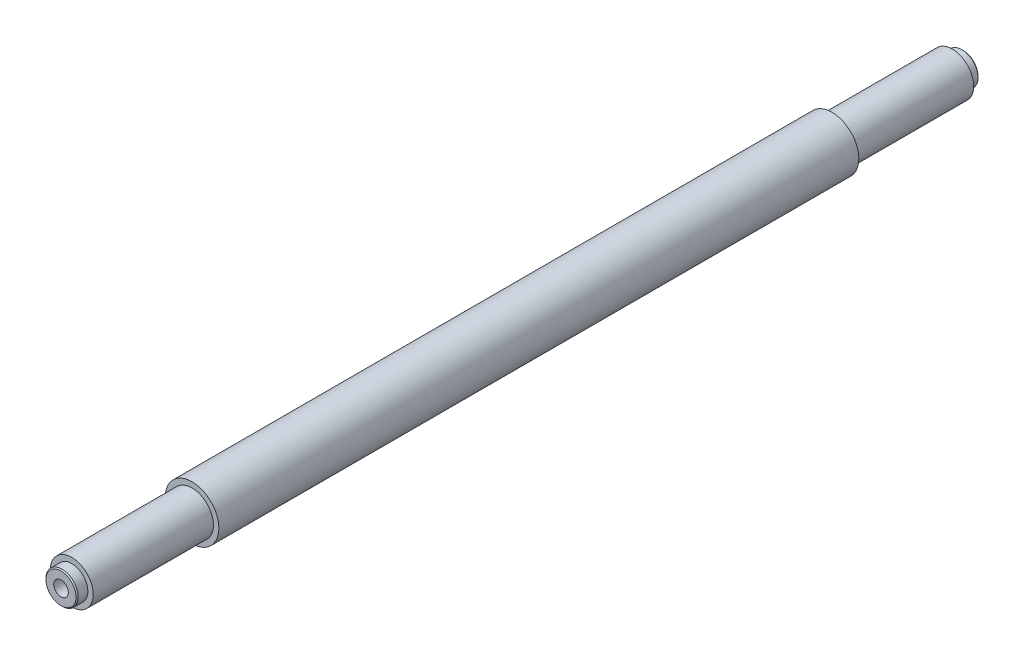
from build123d import *

# Parameters (mm, degrees)
SKETCH_1_R             = 12.5
EXTRUDE_1_DEPTH        = 298
SKETCH_2_R             = 10
EXTRUDE_2_DEPTH        = 56
EXTRUDE_START          = 56
SKETCH_3_R             = 10
EXTRUDE_3_DEPTH        = 56
SKETCH_4_R             = 7.5
EXTRUDE_4_DEPTH        = 5
EXTRUDE_START_2        = 5
SKETCH_5_R             = 7.5
EXTRUDE_5_DEPTH        = 5
HOLE_WIZARD_M8_1_D     = 6.8
HOLE_WIZARD_M8_1_DEPTH = 19.75
HOLE_WIZARD_M8_1_TIP   = 2.042926105
HOLE_WIZARD_M8_2_D     = 6.8
HOLE_WIZARD_M8_2_DEPTH = 19.75
HOLE_WIZARD_M8_2_TIP   = 2.042926105
CHAMFER_2_SIZE         = 0.5
CHAMFER_3_SIZE         = 0.5


with BuildPart() as part:
    # 草图1 → 凸台-拉伸1 (new body)
    with BuildSketch(Plane.XY):
        Circle(SKETCH_1_R)
    extrude(amount=EXTRUDE_1_DEPTH)

    # 草图2 → 凸台-拉伸2 (add)
    with BuildSketch(Plane(origin=(0, 0, 0), x_dir=(-1, 0, 0), z_dir=(0, 0, -1))):
        with Locations(Location((0, 0, 0), (0, 0, 180))):
            Circle(SKETCH_2_R)
    extrude(amount=EXTRUDE_2_DEPTH)

    # 草图3 → 凸台-拉伸3 (add)
    with BuildSketch(Plane.XY.offset(298).offset(EXTRUDE_START)):
        Circle(SKETCH_3_R)
    extrude(amount=-EXTRUDE_3_DEPTH)

    # 草图4 → 凸台-拉伸4 (add)
    with BuildSketch(Plane.XY.offset(354)):
        Circle(SKETCH_4_R)
    extrude(amount=EXTRUDE_4_DEPTH)

    # 草图5 → 凸台-拉伸5 (add)
    with BuildSketch(Plane(origin=(0, 0, -56), x_dir=(-1, 0, 0), z_dir=(0, 0, -1)).offset(EXTRUDE_START_2)):
        with Locations(Location((0, 0, 0), (0, 0, 180))):
            Circle(SKETCH_5_R)
    extrude(amount=-EXTRUDE_5_DEPTH)

    # M8 螺纹孔1
    with Locations(Plane(origin=(0, 0, -61), x_dir=(-1, 0, 0), z_dir=(0, 0, -1))):
        with Locations((0, 0)):
            Hole(HOLE_WIZARD_M8_1_D / 2, depth=HOLE_WIZARD_M8_1_DEPTH)
            with Locations((0, 0, -(HOLE_WIZARD_M8_1_DEPTH + HOLE_WIZARD_M8_1_TIP / 2))):  # 118° drill point
                Cone(0, HOLE_WIZARD_M8_1_D / 2, HOLE_WIZARD_M8_1_TIP, mode=Mode.SUBTRACT)

    # M8 螺纹孔2
    with Locations(Plane.XY.offset(359)):
        with Locations((0, 0)):
            Hole(HOLE_WIZARD_M8_2_D / 2, depth=HOLE_WIZARD_M8_2_DEPTH)
            with Locations((0, 0, -(HOLE_WIZARD_M8_2_DEPTH + HOLE_WIZARD_M8_2_TIP / 2))):  # 118° drill point
                Cone(0, HOLE_WIZARD_M8_2_D / 2, HOLE_WIZARD_M8_2_TIP, mode=Mode.SUBTRACT)

    # 倒角2
    chamfer_2_edges = [part.edges().sort_by_distance(p)[0] for p in [
        (-7.5, 0, 359),
    ]]
    chamfer(chamfer_2_edges, length=CHAMFER_2_SIZE)

    # 倒角3
    chamfer_3_edges = [part.edges().sort_by_distance(p)[0] for p in [
        (-7.5, 0, -61),
    ]]
    chamfer(chamfer_3_edges, length=CHAMFER_3_SIZE)


solid = part.part
